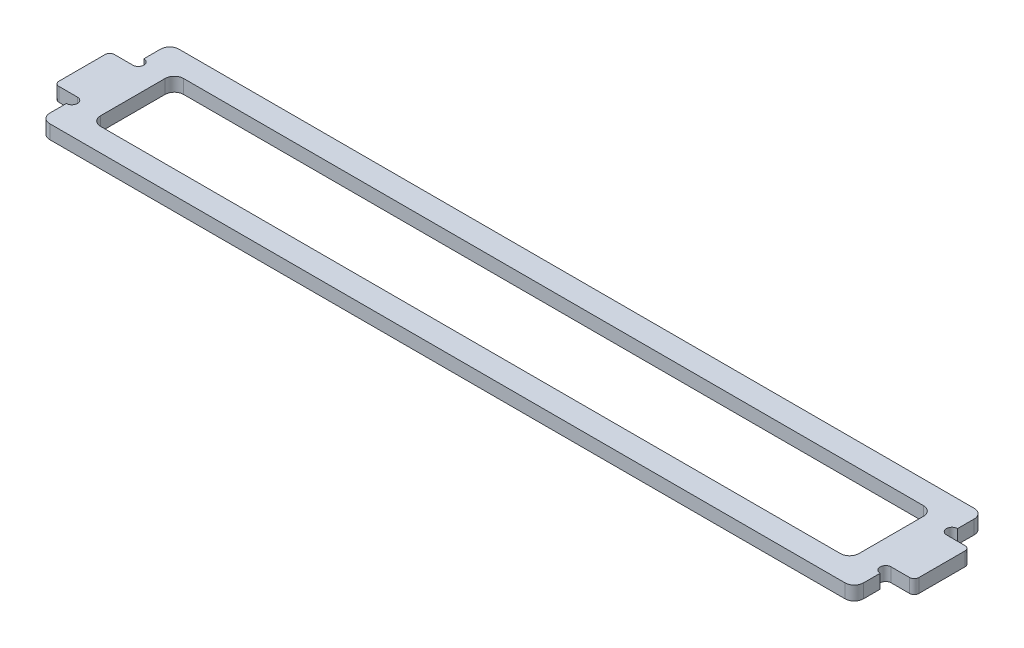
from build123d import *

# Parameters (mm, degrees)
SKETCH_1_W      = 82.2
SKETCH_1_H      = 9
EXTRUDE_1_DEPTH = 1.5
FILLET_1_R      = 0.5
FILLET_2_R      = 1


with BuildPart() as part:
    # 草图1 → 凸台-拉伸1 (new body)
    with BuildSketch(Plane(origin=(0, 0, 0), x_dir=(1, 0, 0), z_dir=(0, 1, 0))):
        with BuildLine():
            Line((44.1, 7), (-44.1, 7))
            Line((-44.1, 7), (-44.1, 4.2))
            ThreePointArc((-44.1, 4.2), (-43.5, 3.6), (-44.1, 3))
            Line((-44.1, 3), (-46.6, 3))
            Line((-46.6, 3), (-46.6, -3))
            Line((-46.6, -3), (-44.1, -3))
            ThreePointArc((-44.1, -3), (-43.5, -3.6), (-44.1, -4.2))
            Line((-44.1, -4.2), (-44.1, -7))
            Line((-44.1, -7), (44.1, -7))
            Line((44.1, -7), (44.1, -4.2))
            ThreePointArc((44.1, -4.2), (43.5, -3.6), (44.1, -3))
            Line((44.1, -3), (46.6, -3))
            Line((46.6, -3), (46.6, 3))
            Line((46.6, 3), (44.1, 3))
            ThreePointArc((44.1, 3), (43.5, 3.6), (44.1, 4.2))
            Line((44.1, 4.2), (44.1, 7))
        make_face()
        Rectangle(SKETCH_1_W, SKETCH_1_H, mode=Mode.SUBTRACT)
    extrude(amount=EXTRUDE_1_DEPTH)

    # 圆角1
    fillet_1_edges = [part.edges().sort_by_distance(p)[0] for p in [
        (46.6, 0.75, -3),
        (46.6, 0.75, 3),
        (-46.6, 0.75, 3),
        (-46.6, 0.75, -3),
    ]]
    fillet(fillet_1_edges, radius=FILLET_1_R)

    # 圆角2
    fillet_2_edges = [part.edges().sort_by_distance(p)[0] for p in [
        (-44.1, 0.75, -7),
        (44.1, 0.75, -7),
        (44.1, 0.75, 7),
        (-44.1, 0.75, 7),
        (-41.1, 0.75, -4.5),
        (-41.1, 0.75, 4.5),
        (41.1, 0.75, 4.5),
        (41.1, 0.75, -4.5),
    ]]
    fillet(fillet_2_edges, radius=FILLET_2_R)


solid = part.part
